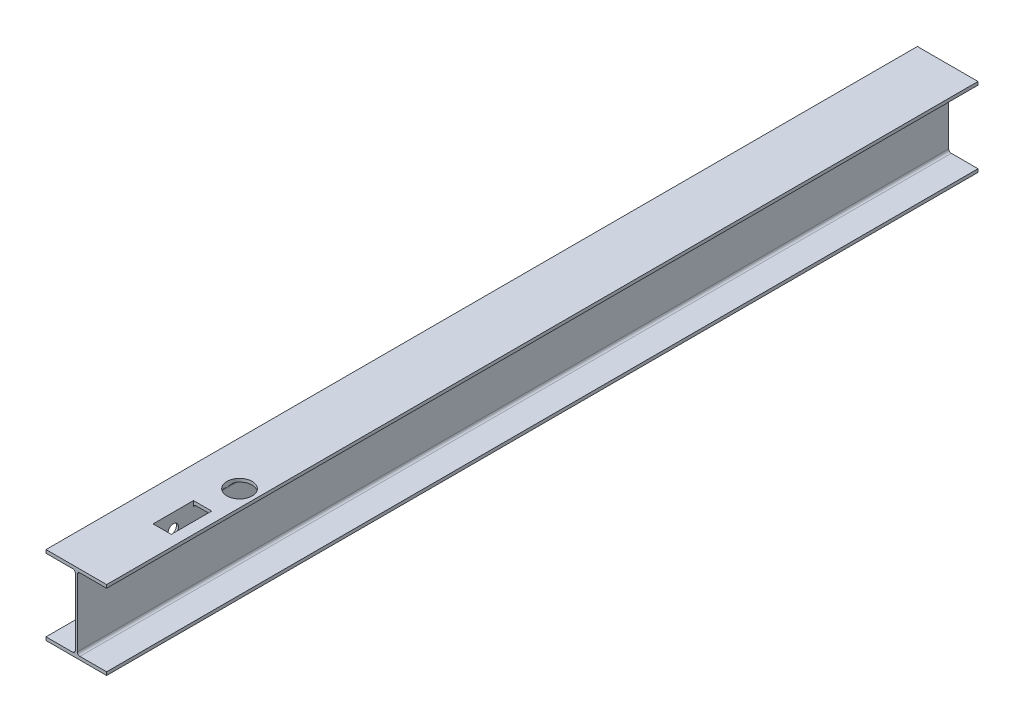
SolidWorks part; units mm, degrees
material "Q235"
ref_plane "Front Plane" through (0, 0, 0) normal (0, 0, 1) x (1, 0, 0)
ref_plane "Top Plane" through (0, 0, 0) normal (0, 1, 0) x (1, 0, 0)
ref_plane "Right Plane" through (0, 0, 0) normal (1, 0, 0) x (0, 0, -1)
sketch "Sketch1" plane through (0, 0, 0) normal (0, 0, 1) x (1, 0, 0)
  line L0 (0, 0) -> (300, 0)
  line L1 (300, 0) -> (300, 16)
  line L2 (300, 16) -> (168, 16)
  line L3 (155, 29) -> (155, 361)
  line L4 (168, 374) -> (300, 374)
  line L5 (300, 374) -> (300, 390)
  line L6 (300, 390) -> (0, 390)
  line L7 (0, 390) -> (0, 374)
  line L8 (0, 374) -> (132, 374)
  line L9 (145, 361) -> (145, 29)
  line L10 (132, 16) -> (0, 16)
  line L11 (0, 16) -> (0, 0)
  line L12 (150, 390) -> (150, 0) construction
  arc A0 (168, 16) -> (155, 29) centre (168, 29) cw
  arc A1 (145, 29) -> (132, 16) centre (132, 29) cw
  arc A2 (155, 361) -> (168, 374) centre (168, 361) cw
  arc A3 (132, 374) -> (145, 361) centre (132, 361) cw
  point P21 (155, 374)
  dimension "D7" = 13
  dimension "D1" = 390
  dimension "D2" = 300
  dimension "D3" = 10
  dimension "D4" = 5
  dimension "D5" = 16
  dimension "D6" = 16
extrude "Boss-Extrude1" add sketch "Sketch1" along normal blind 4313
sketch "Sketch2" plane through (0, 390, 0) normal (0, 1, 0) x (1, 0, 0)
  line L0 (300, -4313) -> (300, 0) construction
  line L1 (245, -3738) -> (155, -3738)
  line L2 (245, -3738) -> (245, -3938)
  line L3 (245, -3938) -> (155, -3938)
  line L4 (155, -3738) -> (155, -3938)
  line L5 (300, -4313) -> (0, -4313) construction
  line L6 (155, -4313) -> (155, 0) construction
  circle A0 centre (218, -3573) radius 62.5
  dimension "D1" = 125
  dimension "D4" = 82
  dimension "D5" = 375
  dimension "D7" = 365
  dimension "D2" = 200
  dimension "D3" = 90
  dimension "D6" = 0
extrude "Cut-Extrude1" cut sketch "Sketch2" against normal up to next
sketch "Sketch3" plane through (155, 0, 0) normal (1, 0, 0) x (0, 0, -1)
  line L0 (-4313, 29) -> (-4313, 361) construction
  line L1 (-3738, 390) -> (-3938, 390) construction
  circle A0 centre (-3838, 315) radius 25.5
  dimension "D1" = 51
  dimension "D2" = 475
  dimension "D3" = 75
extrude "Cut-Extrude2" cut sketch "Sketch3" against normal up to next
